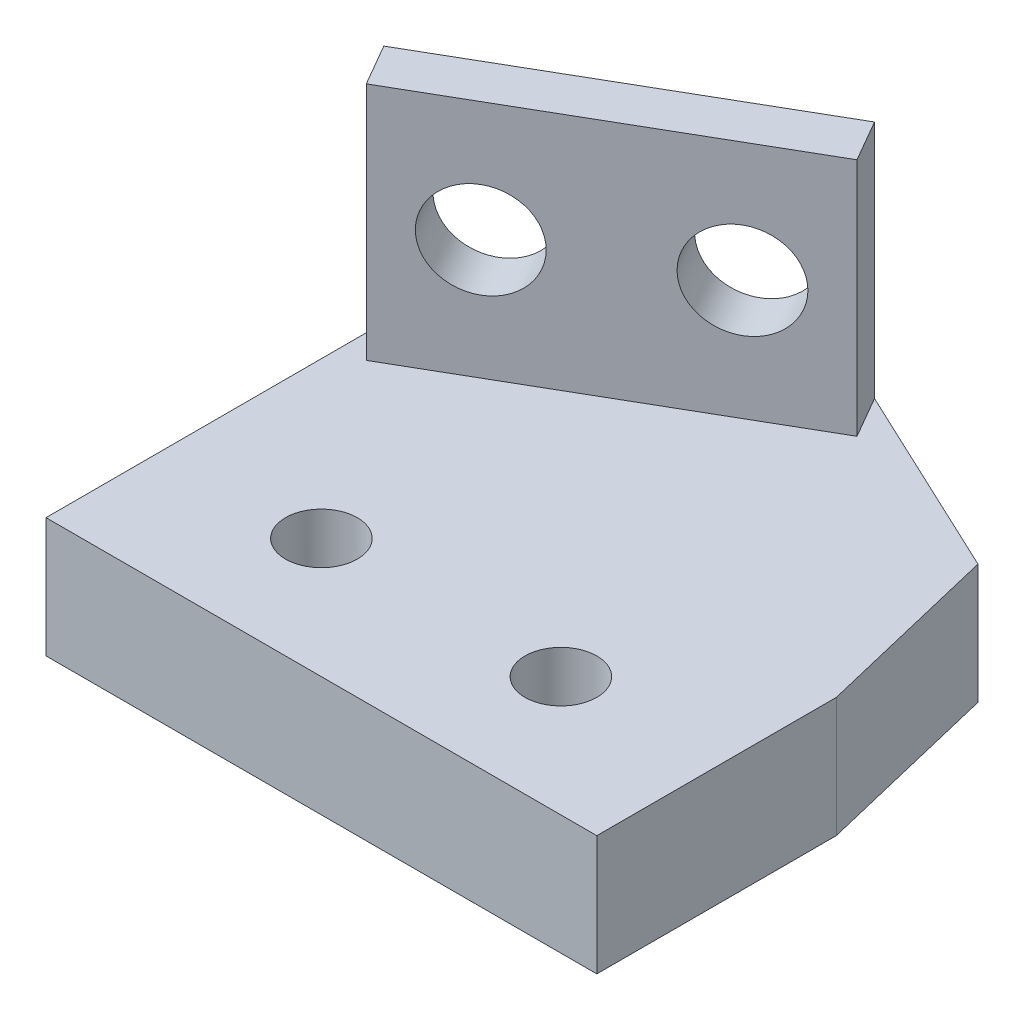
from build123d import *

# Parameters (mm, degrees)
BOSS_EXTRUDE1_DEPTH     = 5
BOSS_EXTRUDE2_DEPTH     = 10
CUT_EXTRUDE1_DEPTH      = 27.946503772
CUT_EXTRUDE1_DEPTH_BACK = 27.946503772
SKETCH3_R               = 2
CUT_EXTRUDE2_DEPTH      = 34.102948638
CUT_EXTRUDE2_DEPTH_BACK = 34.102948638
SKETCH4_R               = 1.5


with BuildPart() as part:
    # Sketch1 → Boss-Extrude1 (new body)
    with BuildSketch(Plane(origin=(0, 0, 0), x_dir=(1, 0, 0), z_dir=(0, 1, 0))):
        Polygon((0, 0), (-23, 0), (-23, 14.105675379), (-10.009618943, 21.605675379), (-1.863192499, 17.780007308), (0, 10), align=None)
    extrude(amount=BOSS_EXTRUDE1_DEPTH)

    # Sketch2 → Boss-Extrude2 (add)
    with BuildSketch(Plane(origin=(0, 5, 0), x_dir=(1, 0, 0), z_dir=(0, 1, 0))):
        Polygon((-22, 12.373624571), (-9.009618943, 19.873624571), (-10.009618943, 21.605675379), (-23, 14.105675379), align=None)
    extrude(amount=BOSS_EXTRUDE2_DEPTH)

    # Sketch3 → Cut-Extrude1 (cut, two sides: drawn at the far end of the back side and taken through both)
    with BuildSketch(Plane(origin=(-10.857936608, 0, -18.80649787), x_dir=(0.8660254037844384, 0, -0.5000000000000004), z_dir=(0.5000000000000004, 0, 0.8660254037844384)).offset(-CUT_EXTRUDE1_DEPTH_BACK)):
        with Locations((-9.365746598, 10)):
            Circle(SKETCH3_R)
        with Locations((-1.365746598, 10)):
            Circle(SKETCH3_R)
    extrude(amount=CUT_EXTRUDE1_DEPTH + CUT_EXTRUDE1_DEPTH_BACK, mode=Mode.SUBTRACT)

    # Sketch4 → Cut-Extrude2 (cut, two sides: drawn at the far end of the back side and taken through both)
    with BuildSketch(Plane(origin=(0, 5, 0), x_dir=(1, 0, 0), z_dir=(0, 1, 0)).offset(-CUT_EXTRUDE2_DEPTH_BACK)):
        with Locations(Location((-16.5, 5, 0), (0, 0, 270))):
            Circle(SKETCH4_R)
        with Locations(Location((-6.5, 5, 0), (0, 0, 270))):
            Circle(SKETCH4_R)
    extrude(amount=CUT_EXTRUDE2_DEPTH + CUT_EXTRUDE2_DEPTH_BACK, mode=Mode.SUBTRACT)


solid = part.part
